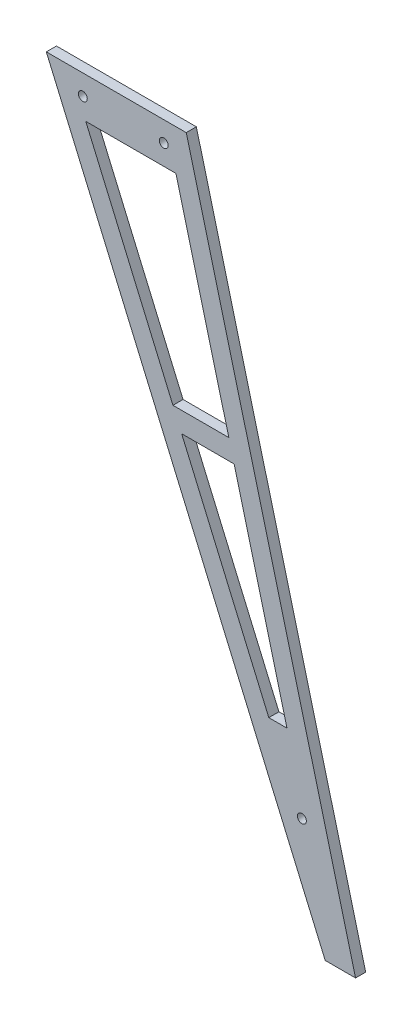
from build123d import *

# Parameters (mm, degrees)
EXTRUDE_1_DEPTH     = 2.5
SKETCH_3_R          = 2.2
CUT_EXTRUDE_1_DEPTH = 10
CUT_EXTRUDE_2_DEPTH = 10
SKETCH_5_R          = 2.2
CUT_EXTRUDE_3_DEPTH = 10


with BuildPart() as part:
    # 草图1 → 凸台-拉伸1 (new, symmetric)
    with BuildSketch(Plane.XY):
        Polygon((255, -663), (171.307692308, -343), (102.153846154, -343), (240, -663), align=None)
    extrude(amount=EXTRUDE_1_DEPTH, both=True)

    # 草图3 → 切除-拉伸1 (cut)
    with BuildSketch(Plane.XY.offset(2.5)):
        with Locations((120.192307692, -353)):
            Circle(SKETCH_3_R)
        with Locations((160.192307692, -353)):
            Circle(SKETCH_3_R)
    extrude(amount=-CUT_EXTRUDE_1_DEPTH, mode=Mode.SUBTRACT)

    # 草图4 → 切除-拉伸2 (cut)
    with BuildSketch(Plane.XY.offset(2.5)):
        Polygon((166.202106442, -363), (121.657582941, -363), (164.734506018, -463), (192.355952596, -463), align=None)
        Polygon((194.971337211, -473), (169.042198326, -473), (212.119121403, -573), (221.125183365, -573), align=None)
    extrude(amount=-CUT_EXTRUDE_2_DEPTH, mode=Mode.SUBTRACT)

    # 草图5 → 切除-拉伸3 (cut)
    with BuildSketch(Plane.XY.offset(2.5)):
        with Locations((228.461538462, -608)):
            Circle(SKETCH_5_R)
    extrude(amount=-CUT_EXTRUDE_3_DEPTH, mode=Mode.SUBTRACT)


solid = part.part
